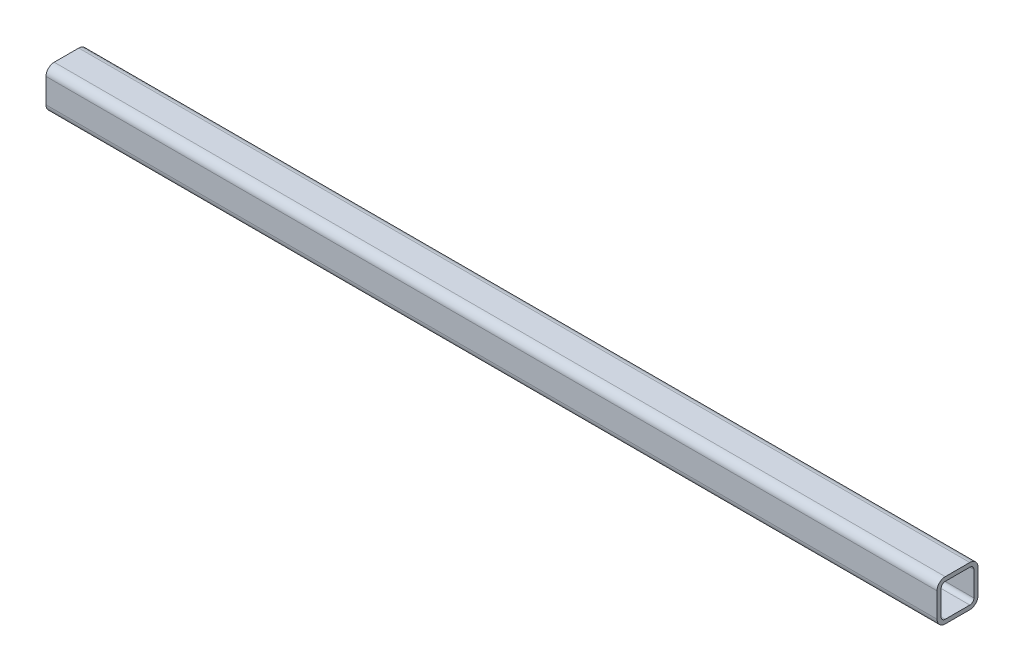
from build123d import *

# Parameters (mm, degrees)
SQUARE_TUBE_40_X_40_X_4_1_DEPTH = 870


with BuildPart() as part:
    # Sketch1 → Square Tube 40 X 40 X 4(1) (new body)
    with BuildSketch(Plane.YZ.offset(-1000)):
        with BuildLine():
            Line((-12, -20), (12, -20))
            ThreePointArc((12, -20), (17.656854249, -17.656854249), (20, -12))
            Line((20, -12), (20, 12))
            ThreePointArc((20, 12), (17.656854249, 17.656854249), (12, 20))
            Line((12, 20), (-12, 20))
            ThreePointArc((-12, 20), (-17.656854249, 17.656854249), (-20, 12))
            Line((-20, 12), (-20, -12))
            ThreePointArc((-20, -12), (-17.656854249, -17.656854249), (-12, -20))
        make_face()
        with BuildLine():
            Line((-12, -16), (12, -16))
            ThreePointArc((12, -16), (14.828427125, -14.828427125), (16, -12))
            Line((16, -12), (16, 12))
            ThreePointArc((16, 12), (14.828427125, 14.828427125), (12, 16))
            Line((12, 16), (-12, 16))
            ThreePointArc((-12, 16), (-14.828427125, 14.828427125), (-16, 12))
            Line((-16, 12), (-16, -12))
            ThreePointArc((-16, -12), (-14.828427125, -14.828427125), (-12, -16))
        make_face(mode=Mode.SUBTRACT)
    extrude(amount=SQUARE_TUBE_40_X_40_X_4_1_DEPTH)


solid = part.part
